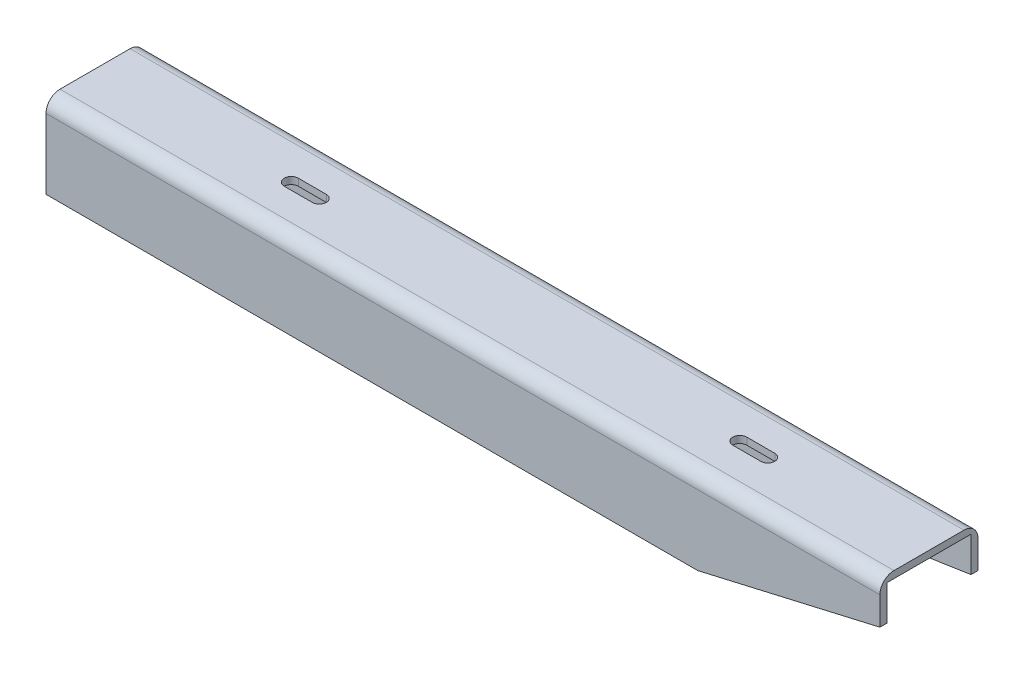
from build123d import *

# Parameters (mm, degrees)
EXTRUDE_1_DEPTH     = 70
SHELL_1_T           = -5
EXTRUDE_2_DEPTH     = 5
CUT_EXTRUDE_1_DEPTH = 5
FILLET_1_R          = 10
FILLET_2_R          = 10
CUT_EXTRUDE_2_DEPTH = 5


with BuildPart() as part:
    # 草图1 → 凸台-拉伸1 (new body)
    with BuildSketch(Plane.XY):
        Polygon((0, 70), (0, -50), (595, 40), (595, 70), (570, 70), align=None)
    extrude(amount=EXTRUDE_1_DEPTH)

    # 抽壳1
    shell_1_openings = [part.faces().sort_by_distance(p)[0] for p in [
        (0, 10, 35),
        (595, 55, 35),
        (297.5, -5, 35),
    ]]
    offset(amount=SHELL_1_T, openings=shell_1_openings, kind=Kind.INTERSECTION)

    # 草图2 → 凸台-拉伸2 (add)
    with BuildSketch(Plane.XY.offset(70)):
        Polygon((465, 10), (595, 40), (396.666666667, 10), align=None)
    extrude(amount=-EXTRUDE_2_DEPTH)

    # 草图3 → 切除-拉伸1 (cut)
    with BuildSketch(Plane.XY.offset(70)):
        Polygon((0, -50), (396.666666667, 10), (0, 10), align=None)
    extrude(amount=-CUT_EXTRUDE_1_DEPTH, mode=Mode.SUBTRACT)

    # 圆角1
    fillet_1_edges = [part.edges().sort_by_distance(p)[0] for p in [
        (297.5, 70, 70),
    ]]
    fillet(fillet_1_edges, radius=FILLET_1_R)

    # 圆角2
    fillet_2_edges = [part.edges().sort_by_distance(p)[0] for p in [
        (297.5, 70, 0),
    ]]
    fillet(fillet_2_edges, radius=FILLET_2_R)

    # 草图4 → 切除-拉伸2 (cut)
    with BuildSketch(Plane(origin=(0, 70, 0), x_dir=(1, 0, 0), z_dir=(0, 1, 0))):
        with BuildLine():
            Line((160, -40), (140, -40))
            ThreePointArc((140, -40), (135, -35), (140, -30))
            Line((140, -30), (160, -30))
            ThreePointArc((160, -30), (165, -35), (160, -40))
        make_face()
        with BuildLine():
            Line((460, -30), (480, -30))
            ThreePointArc((480, -30), (485, -35), (480, -40))
            Line((480, -40), (460, -40))
            ThreePointArc((460, -40), (455, -35), (460, -30))
        make_face()
    extrude(amount=-CUT_EXTRUDE_2_DEPTH, mode=Mode.SUBTRACT)


solid = part.part
